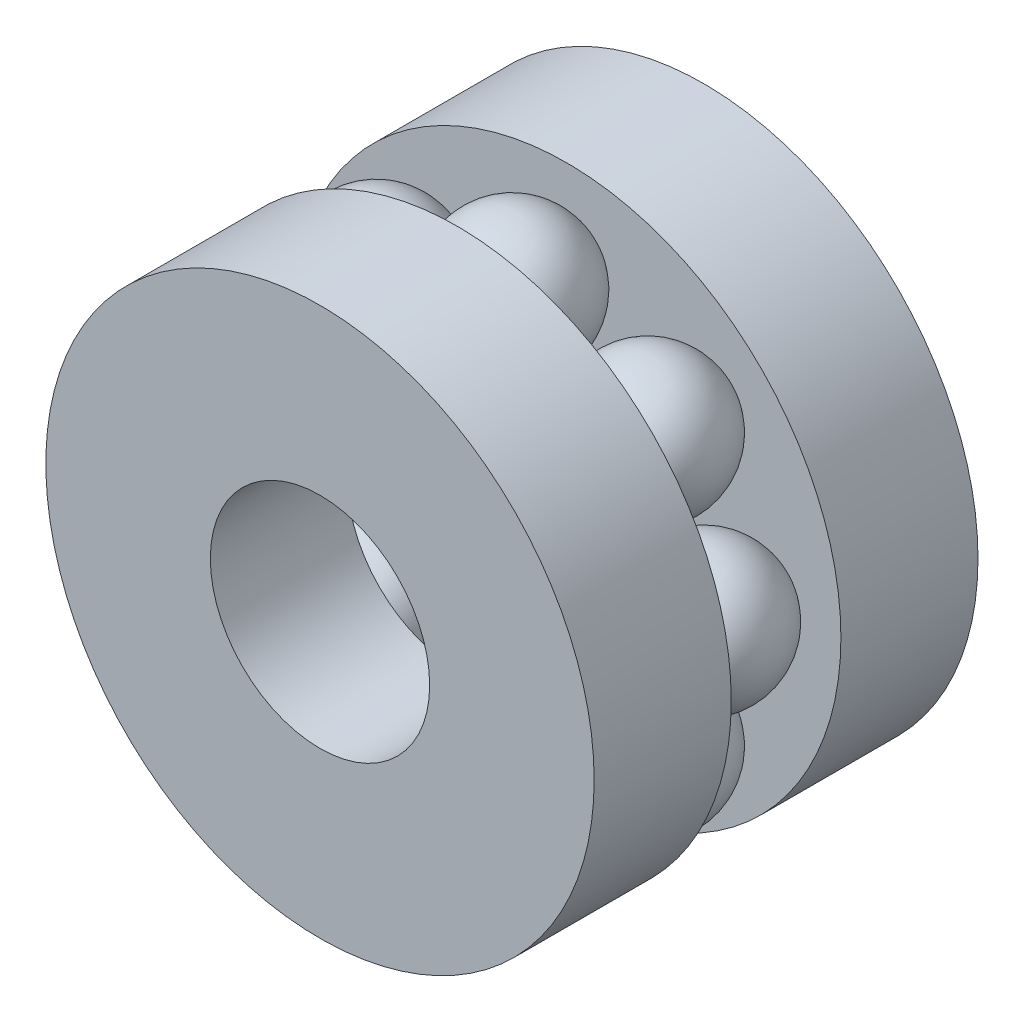
SolidWorks part; units mm, degrees
ref_plane "Front Plane" through (0, 0, 0) normal (0, 0, 1) x (1, 0, 0)
ref_plane "Top Plane" through (0, 0, 0) normal (0, 1, 0) x (1, 0, 0)
ref_plane "Right Plane" through (0, 0, 0) normal (1, 0, 0) x (0, 0, -1)
other "Configuration Table"
sketch "Sketch1" plane through (0, 0, 0) normal (0, 0, 1) x (1, 0, 0)
  circle A0 centre (0, 0) radius 4
  circle A1 centre (0, 0) radius 10
  dimension "D1" = 8
  dimension "D2" = 20
extrude "Boss-Extrude1" add sketch "Sketch1" along normal blind 5 from offset 5
sketch "Sketch2" plane through (0, 0, 0) normal (1, 0, 0) x (0, 0, -1)
  line L1 (-3, 4.5) -> (-3, 9.5)
  line L2 (0, 0) -> (-18.0499, 0) construction
  arc A0 (-3, 9.5) -> (-3, 4.5) centre (-3, 7) ccw
  dimension "D1" = 5
  dimension "D2" = 7
  dimension "D3" = 3
revolve "Revolve1" add sketch "Sketch2" angle 360 about L1
pattern_circular "CirPattern2" count 8 over 360 about axis through (0, 0, 0) along (0, 0, 1) of "Revolve1"
sketch "Sketch3" plane through (0, 0, 0) normal (0, 0, 1) x (1, 0, 0)
  circle A0 centre (0, 0) radius 10 construction
  circle A1 centre (0, 0) radius 10
  circle A2 centre (0, 0) radius 4 construction
  circle A3 centre (0, 0) radius 4
extrude "Boss-Extrude2" add sketch "Sketch3" against normal blind 5 from offset 1
